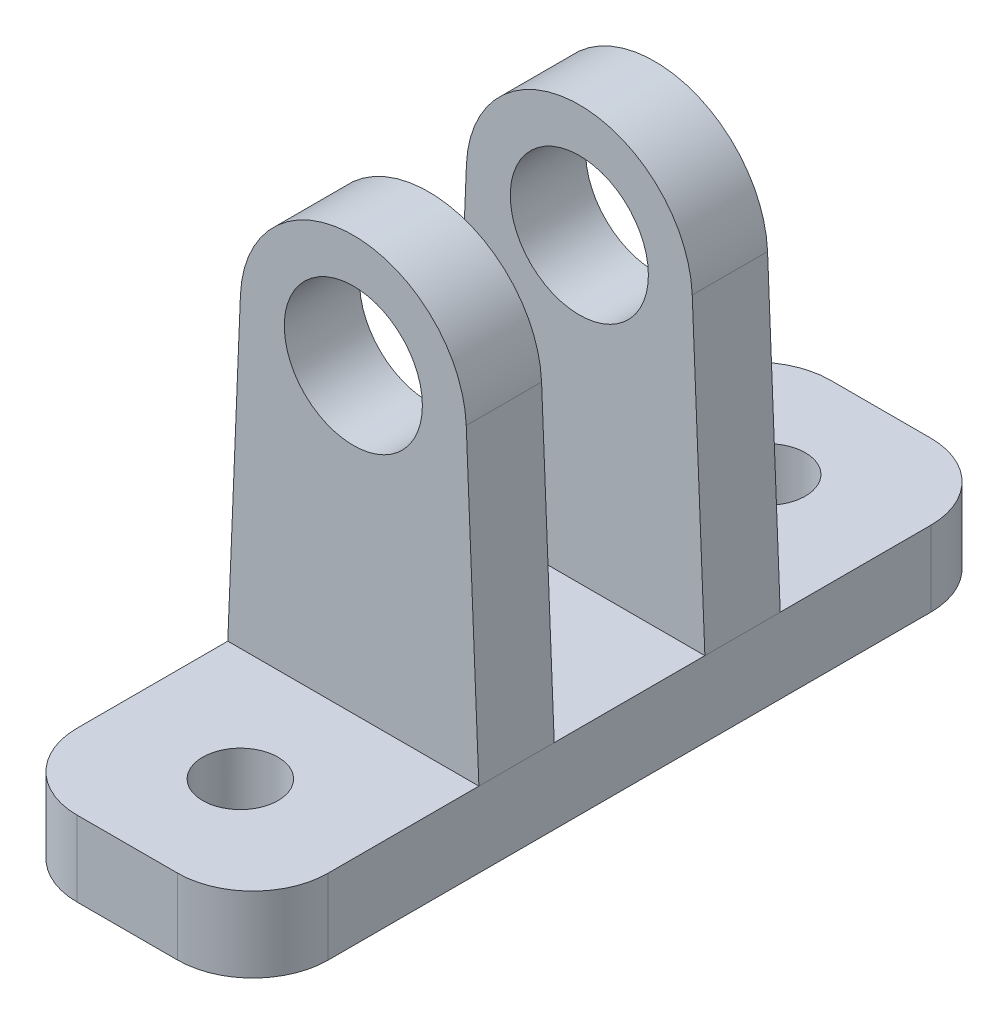
SolidWorks part; units mm, degrees
ref_plane "Front Plane" through (0, 0, 0) normal (0, 0, 1) x (1, 0, 0)
ref_plane "Top Plane" through (0, 0, 0) normal (0, 1, 0) x (1, 0, 0)
ref_plane "Right Plane" through (0, 0, 0) normal (1, 0, 0) x (0, 0, -1)
sketch "Sketch 1" plane through (0, 0, 0) normal (0, 1, 0) x (1, 0, 0)
  line L1 (-50, -60) -> (50, -60)
  line L2 (-50, -60) -> (-50, 60)
  line L3 (-50, 60) -> (50, 60)
  line L4 (50, -60) -> (50, 60)
  line L5 (-50, -60) -> (50, 60) construction
  line L6 (-50, 60) -> (50, -60) construction
  point P0 (0, 0)
  dimension "D1" = 100
  dimension "D2" = 120
extrude "Boss-Extrude 1" add sketch "Sketch 1" along normal blind 30
sketch "Sketch 2" plane through (0, 0, 60) normal (0, 0, 1) x (1, 0, 0)
  line L0 (0, -7.9075) -> (0, 168.2922) construction
  line L1 (-50, 0) -> (50, 0) construction
  line L2 (-44.9616, 151.859) -> (-50, 30)
  line L3 (-50, 30) -> (50, 30) construction
  line L4 (-50, 30) -> (-50, 0) construction
  line L5 (-50, 30) -> (50, 30)
  line L6 (44.9616, 151.859) -> (50, 30)
  circle A0 centre (0, 150) radius 27.5
  arc A1 (44.9616, 151.859) -> (-44.9616, 151.859) centre (0, 150) ccw
  point P17 (0, 30)
  dimension "D1" = 55
  dimension "D2" = 150
  dimension "D3" = 45
extrude "Boss-Extrude 2" add sketch "Sketch 2" against normal blind 30
sketch "Sketch 4" plane through (0, 0, 60) normal (0, 0, 1) x (1, 0, 0)
  line L0 (0, -12.2336) -> (0, 150.8827) construction
  line L1 (-50, 0) -> (50, 0) construction
  line L2 (-7.5, 30) -> (7.5, 30)
  line L3 (-7.5, 30) -> (-7.5, 0)
  line L4 (-7.5, 0) -> (7.5, 0)
  line L5 (7.5, 30) -> (7.5, 0)
  line L6 (-7.5, 30) -> (7.5, 0) construction
  line L7 (-7.5, 0) -> (7.5, 30) construction
  point P3 (0, 15)
  dimension "D1" = 30
  dimension "15" = 15
extrude "Boss-Extrude 3" add sketch "Sketch 4" along normal blind 30
mirror "Mirror 1" about plane through (0, 0, 0) normal (0, 0, 1) of "Boss-Extrude 2", "Boss-Extrude 3"
sketch "Sketch 5" plane through (0, 0, 0) normal (0, -1, 0) x (1, 0, 0)
  line L0 (-50, -60) -> (-50, 60) construction
  line L1 (50, -150) -> (-50, -150)
  line L2 (50, -150) -> (50, 150)
  line L3 (50, 150) -> (-50, 150)
  line L4 (-50, -150) -> (-50, 150)
  line L5 (50, -150) -> (-50, 150) construction
  line L6 (50, 150) -> (-50, -150) construction
  line L7 (0, -312.6276) -> (0, 307.996) construction
  line L8 (-7.5, -60) -> (-50, -60) construction
  line L9 (-125.9194, -105) -> (134.6035, -105) construction
  line L11 (-132.1053, 0) -> (125.2238, 0) construction
  line L13 (-44.9616, -60) -> (44.9616, -60) construction
  circle A0 centre (0, -105) radius 15
  circle A1 centre (0, 105) radius 15
  point P0 (0, 0)
  dimension "D2" = 30
  dimension "D1" = 90
extrude "Boss-Extrude 4" add sketch "Sketch 5" against normal up to surface (30 mm away) up to face at (0, 30, 0)
fillet "Fillet 1" radius 30 4 edges at (50, 15, 150) (-50, 15, 150) (50, 15, -150) (-50, 15, -150)
